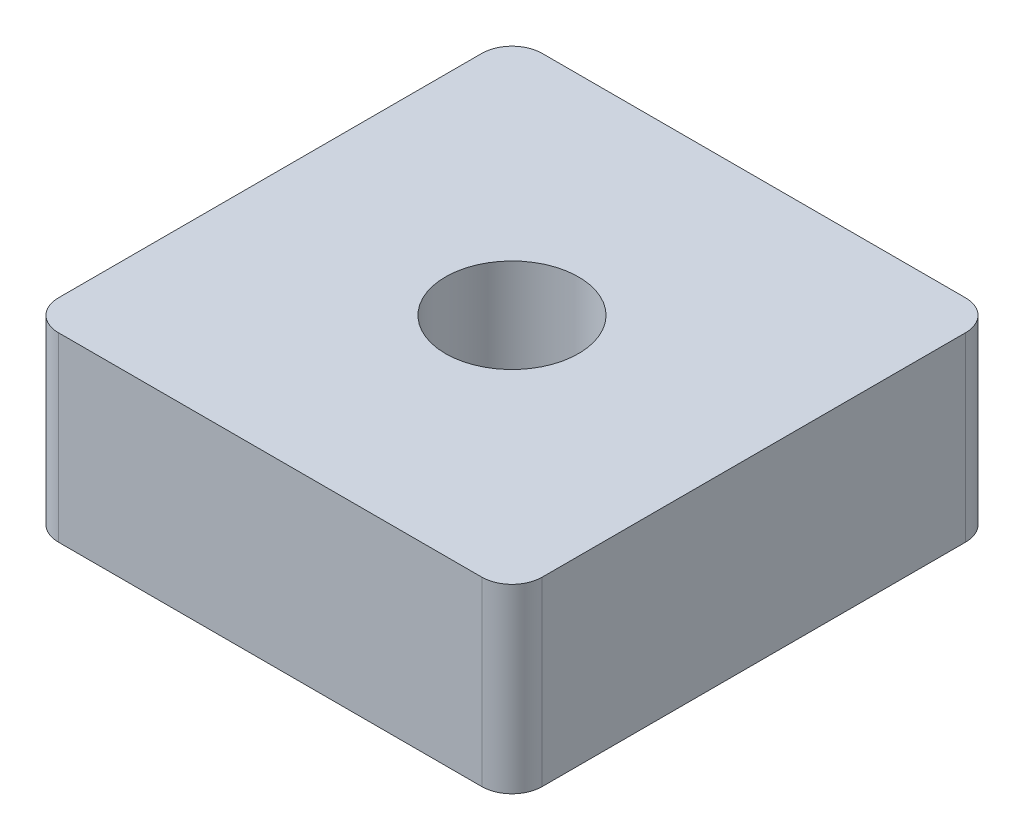
SolidWorks part; units mm, degrees
ref_plane "Front Plane" through (0, 0, 0) normal (0, 0, 1) x (1, 0, 0)
ref_plane "Top Plane" through (0, 0, 0) normal (0, 1, 0) x (1, 0, 0)
ref_plane "Right Plane" through (0, 0, 0) normal (1, 0, 0) x (0, 0, -1)
sketch "Sketch1" plane through (0, 0, 0) normal (0, 1, 0) x (1, 0, 0)
  line L1 (-40, 40) -> (40, 40)
  line L2 (-40, 40) -> (-40, -40)
  line L3 (-40, -40) -> (40, -40)
  line L4 (40, 40) -> (40, -40)
  line L5 (-40, 40) -> (40, -40) construction
  line L6 (-40, -40) -> (40, 40) construction
  point P0 (0, 0)
  dimension "D1" = 80
  dimension "D2" = 80
extrude "Boss-Extrude1" add sketch "Sketch1" along normal blind 30
fillet "Fillet1" radius 5 4 edges at (-40, 15, -40) (40, 15, -40) (40, 15, 40) (-40, 15, 40)
hole_wizard "M24x2.0 Tapped Hole1" positions "Sketch2" profile "Sketch3" tap size "M24x2.0" standard "ANSI Metric" end condition through all
sketch "Sketch2" plane through (0, 30, 0) normal (0, 1, 0) x (1, 0, 0)
  point P0 (0, 0)
sketch "Sketch3" plane through (0, 30, 0) normal (1, 0, 0) x (0, 0, 1)
  line L0 (0, 0) -> (0, 30)
  line L1 (0, 30) -> (11, 30)
  line L2 (11, 30) -> (11, 0)
  line L5 (11, 0) -> (0, 0)
  line L11 (0, -6.35) -> (0, 107.95) construction
  dimension "螺纹线主直径" = 22
  dimension "通孔螺纹孔钻头深度" = 30
